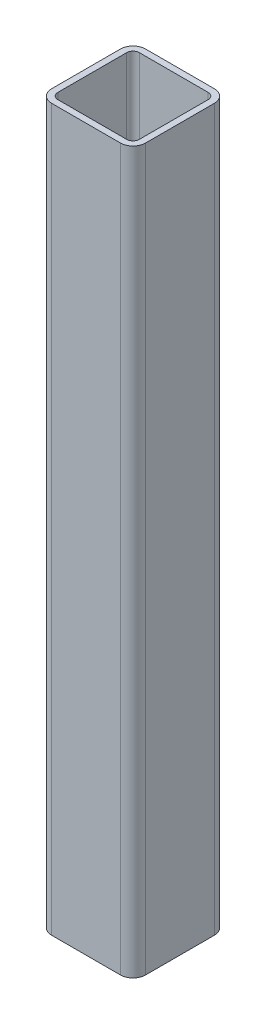
from build123d import *

# Parameters (mm, degrees)
GB_T_6728_2002_SQUARE_HOLLOW_SECTION_30_DEPTH = 230


with BuildPart() as part:
    # Sketch11 → Gb／t 6728—2002 square hollow section 30×30×2(1) (new body)
    with BuildSketch(Plane(origin=(0, 0, 0), x_dir=(-1, 0, 0), z_dir=(0, 1, 0))):
        with BuildLine():
            Line((-11, -15), (11, -15))
            ThreePointArc((11, -15), (13.828427125, -13.828427125), (15, -11))
            Line((15, -11), (15, 11))
            ThreePointArc((15, 11), (13.828427125, 13.828427125), (11, 15))
            Line((11, 15), (-11, 15))
            ThreePointArc((-11, 15), (-13.828427125, 13.828427125), (-15, 11))
            Line((-15, 11), (-15, -11))
            ThreePointArc((-15, -11), (-13.828427125, -13.828427125), (-11, -15))
        make_face()
        with BuildLine():
            Line((-11, -13), (11, -13))
            ThreePointArc((11, -13), (12.414213562, -12.414213562), (13, -11))
            Line((13, -11), (13, 11))
            ThreePointArc((13, 11), (12.414213562, 12.414213562), (11, 13))
            Line((11, 13), (-11, 13))
            ThreePointArc((-11, 13), (-12.414213562, 12.414213562), (-13, 11))
            Line((-13, 11), (-13, -11))
            ThreePointArc((-13, -11), (-12.414213562, -12.414213562), (-11, -13))
        make_face(mode=Mode.SUBTRACT)
    extrude(amount=GB_T_6728_2002_SQUARE_HOLLOW_SECTION_30_DEPTH)


solid = part.part
